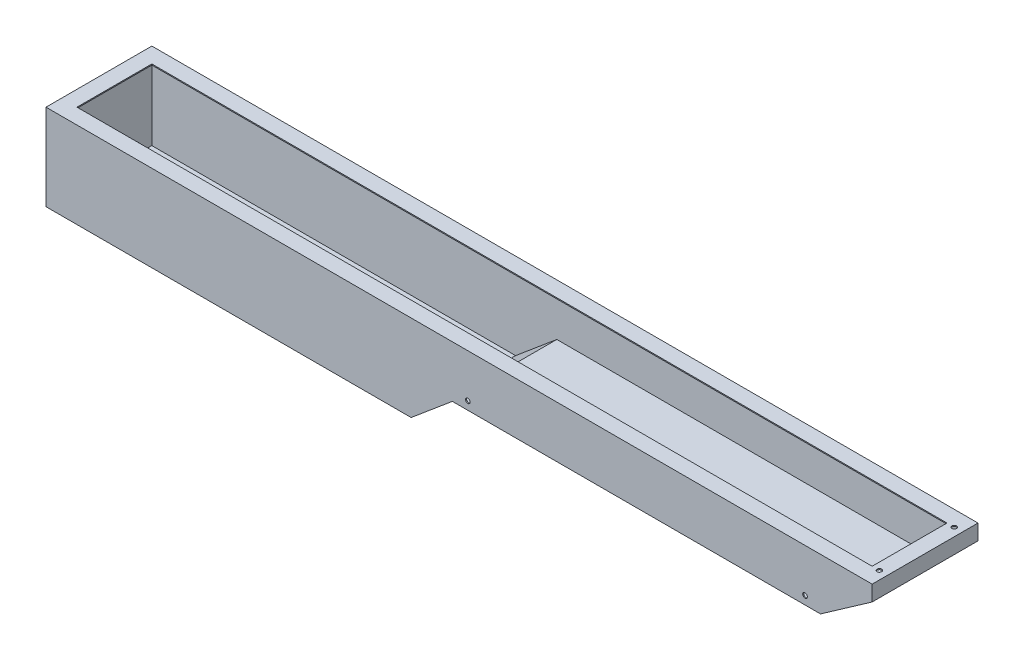
SolidWorks part; units mm, degrees
ref_plane "前视基准面" through (0, 0, 0) normal (0, 0, 1) x (1, 0, 0)
ref_plane "上视基准面" through (0, 0, 0) normal (0, 1, 0) x (1, 0, 0)
ref_plane "右视基准面" through (0, 0, 0) normal (1, 0, 0) x (0, 0, -1)
sketch "草图2" plane through (0, 0, 0) normal (0, 0, -1) x (-1, 0, 0)
  line L0 (0, 0) -> (772.2061, 0) construction
  line L1 (0, 0) -> (0, -417.7577) construction
  line L18 (-1600, -30) -> (-1500.0296, -100)
  line L19 (-1600, 0) -> (-1600, -30)
  line L21 (0, 0) -> (-1600, 0)
  line L23 (0, -167) -> (0, 0)
  line L24 (-707.1525, -167) -> (0, -167)
  line L25 (-787, -100) -> (-707.1525, -167)
  line L26 (-1500.0296, -100) -> (-787, -100)
  dimension "D1" = 167
  dimension "D2" = 813
  dimension "D3" = 145
  dimension "D4" = 30
  dimension "D5" = 1600
  dimension "D7" = 100
  dimension "D11" = 140
extrude "凸台-拉伸1" add sketch "草图2" along normal blind 205
shell "抽壳1" thickness 2
sketch "草图4" plane through (0, 0, 0) normal (0, 1, 0) x (1, 0, 0)
  line L0 (30, 175) -> (30, 30)
  line L1 (0, 205) -> (1600, 205)
  line L2 (0, 205) -> (0, 0)
  line L3 (0, 0) -> (1600, 0)
  line L4 (1600, 205) -> (1600, 0)
  line L5 (30, 30) -> (1570, 30)
  line L6 (1570, 175) -> (1570, 30)
  line L7 (30, 175) -> (1570, 175)
  dimension "D1" = 30
extrude "凸台-拉伸2" add sketch "草图4" against normal blind 2
sketch "草图5" plane through (0, 0, -205) normal (0, 0, -1) x (-1, 0, 0)
  line L1 (0, -167) -> (0, 0) construction
  line L2 (0, -14) -> (-1600, -14)
  line L3 (0, -14) -> (-1600, -14) construction
  line L4 (-1600, 0) -> (-1600, -30) construction
  line L5 (-800, 0) -> (-800, -331.4304) construction
  line L6 (0, 0) -> (-1600, 0) construction
  circle A0 centre (-1570, -14) radius 4.5
  circle A1 centre (-30, -14) radius 4.5
  circle A2 centre (-800, -14) radius 4.5
  dimension "D2" = 9
  dimension "D3" = 9
  dimension "D4" = 30
  dimension "D5" = 30
  dimension "D6" = 9
  dimension "D1" = 14
extrude "切除-拉伸1" cut sketch "草图5" against normal blind 2
sketch "草图7" plane through (0, 0, 0) normal (-1, 0, 0) x (0, 0, 1)
  line L1 (0, -167) -> (0, 0) construction
  line L2 (-205, -151) -> (0, -151)
  line L3 (-205, -151) -> (0, -151) construction
  line L4 (-205, -167) -> (-205, 0) construction
  circle A0 centre (-175, -151) radius 4.5
  circle A1 centre (-30, -151) radius 4.5
  dimension "D2" = 30
  dimension "D3" = 9
  dimension "D4" = 30
  dimension "D5" = 9
  dimension "D1" = 16
extrude "切除-拉伸2" cut sketch "草图7" against normal blind 78
sketch "草图8" plane through (0, 0, 0) normal (0, 1, 0) x (1, 0, 0)
  line L1 (0, 0) -> (1600, 0) construction
  line L2 (1584, 30) -> (1584, 175)
  line L3 (1584, -20.199) -> (1584, 241.0827) construction
  line L4 (0, 205) -> (1600, 205) construction
  circle A0 centre (1584, 175) radius 4.5
  circle A1 centre (1584, 30) radius 4.5
  dimension "D2" = 9
  dimension "D3" = 9
  dimension "D4" = 30
  dimension "D5" = 30
  dimension "D1" = 14
extrude "切除-拉伸3" cut sketch "草图8" against normal blind 16
sketch "草图9" plane through (0, 0, 0) normal (0, 0, 1) x (1, 0, 0)
  line L1 (787, -100) -> (787, 155.6413) construction
  line L2 (1500.0296, -84) -> (787, -84)
  line L3 (1500.0296, -84) -> (787, -84) construction
  line L4 (1500.0296, -100) -> (1500.0296, 136.2787) construction
  line L5 (817, -100) -> (817, 155.6413) construction
  line L6 (1470.0296, -100) -> (1470.0296, 136.2787) construction
  circle A0 centre (817, -84) radius 4.5
  circle A1 centre (1470.0296, -84) radius 4.5
  dimension "D4" = 9
  dimension "D5" = 9
  dimension "D1" = 16
  dimension "D2" = 30
  dimension "D3" = 30
extrude "切除-拉伸4" cut sketch "草图9" against normal blind 110
